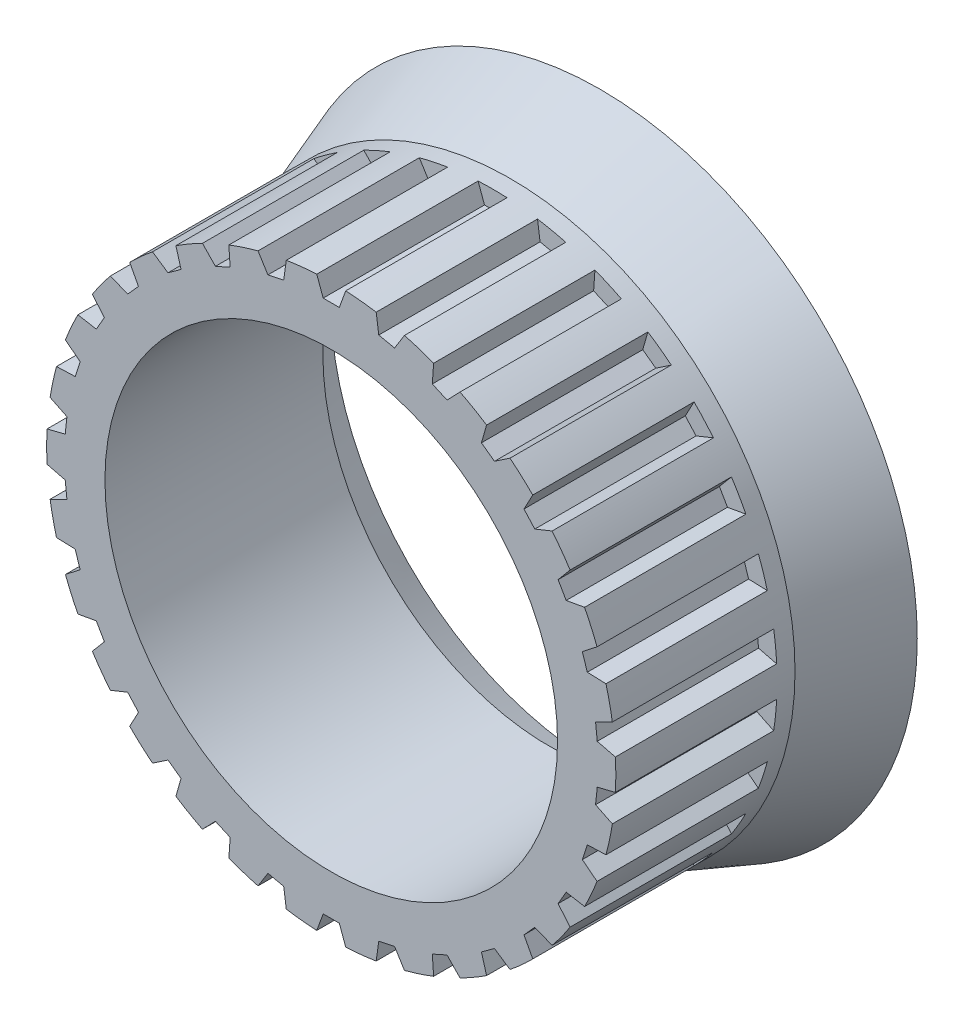
from build123d import *

# Parameters (mm, degrees)
M56_TAPPED_HOLE1_D     = 50.5
M56_TAPPED_HOLE1_DEPTH = 128.5
M56_TAPPED_HOLE1_TIP   = 15.17173063
CUT_EXTRUDE1_DEPTH     = 18
CIRPATTERN1_COUNT      = 30


with BuildPart() as part:
    # Sketch1 → Revolve1 (revolve)
    with BuildSketch(Plane(origin=(0, 0, 0), x_dir=(0, 0, -1), z_dir=(1, 0, 0)), mode=Mode.PRIVATE) as revolve1_sk:
        Polygon((0, 31.75), (0, 0), (24.315981678, 0), (24.315981678, 28), (30, 30.06881348), (30, 35.389702343), (20, 31.75), align=None)
    revolve(revolve1_sk.sketch.rotate(Axis((0, 0, 16.883037514), (0, 0, -1)), 90), axis=Axis((0, 0, 16.883037514), (0, 0, -1)))

    # M56 Tapped Hole1
    with Locations(Plane.XY):
        with Locations((0, 0)):
            Hole(M56_TAPPED_HOLE1_D / 2, depth=M56_TAPPED_HOLE1_DEPTH)
            with Locations((0, 0, -(M56_TAPPED_HOLE1_DEPTH + M56_TAPPED_HOLE1_TIP / 2))):  # 118° drill point
                Cone(0, M56_TAPPED_HOLE1_D / 2, M56_TAPPED_HOLE1_TIP, mode=Mode.SUBTRACT)

    # Sketch6 → Cut-Extrude1 (cut)
    with BuildSketch(Plane.XY):
        with BuildLine():
            Line((0, -31.75), (0, -29.75))
            Line((0, -29.75), (-0.9, -29.75))
            Line((-0.9, -29.75), (-1.613017649, -31.708999891))
            ThreePointArc((-1.613017649, -31.708999891), (-0.80676932, -31.739748318), (0, -31.75))
        make_face()
        with BuildLine():
            Line((0.9, -29.75), (0, -29.75))
            Line((0, -29.75), (0, -31.75))
            ThreePointArc((0, -31.75), (0.80676932, -31.739748318), (1.613017649, -31.708999891))
            Line((1.613017649, -31.708999891), (0.9, -29.75))
        make_face()
    cut_extrude1 = extrude(amount=-CUT_EXTRUDE1_DEPTH, mode=Mode.SUBTRACT)

    # CirPattern1: Cut-Extrude1 ×30 about axis
    cirpattern1_axis = Axis((0, 0, 0), (0, 0, 1))
    for i in range(1, CIRPATTERN1_COUNT):
        add(cut_extrude1.rotate(cirpattern1_axis, i * 360 / CIRPATTERN1_COUNT), mode=Mode.SUBTRACT)


solid = part.part
